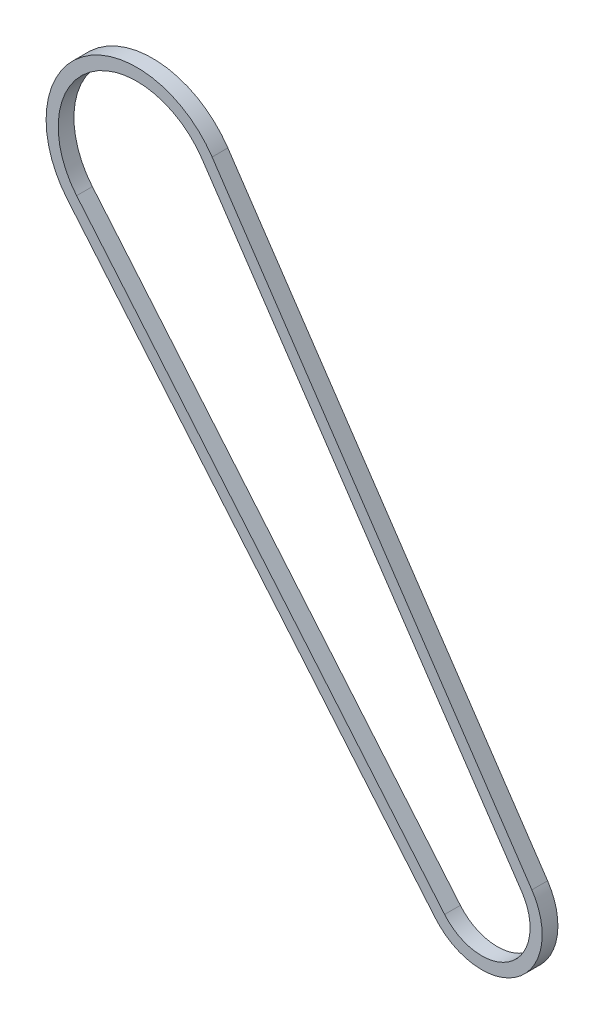
SolidWorks part; units mm, degrees
material "45+钨钢 "
ref_plane "Front Plane" through (0, 0, 0) normal (0, 0, 1) x (1, 0, 0)
ref_plane "Top Plane" through (0, 0, 0) normal (0, 1, 0) x (1, 0, 0)
ref_plane "Right Plane" through (0, 0, 0) normal (1, 0, 0) x (0, 0, -1)
sketch "Sketch2" plane through (0, 0, 0) normal (0, 0, 1) x (1, 0, 0)
  line L0 (0, 0) -> (1, 0) construction
  line L1 (0, 0) -> (0, 1) construction
  line L2 (62.2094, 41.8926) -> (326.473, -350.5323)
  line L3 (246.7014, -410.6044) -> (-57.448, -48.2155)
  arc A0 (-57.448, -48.2155) -> (62.2094, 41.8926) centre (0, 0) cw
  arc A1 (326.473, -350.5323) -> (246.7014, -410.6044) centre (285, -378.4607) cw
extrude "Extrude-Thin1" add sketch "Sketch2" along normal mid plane 13 thin
